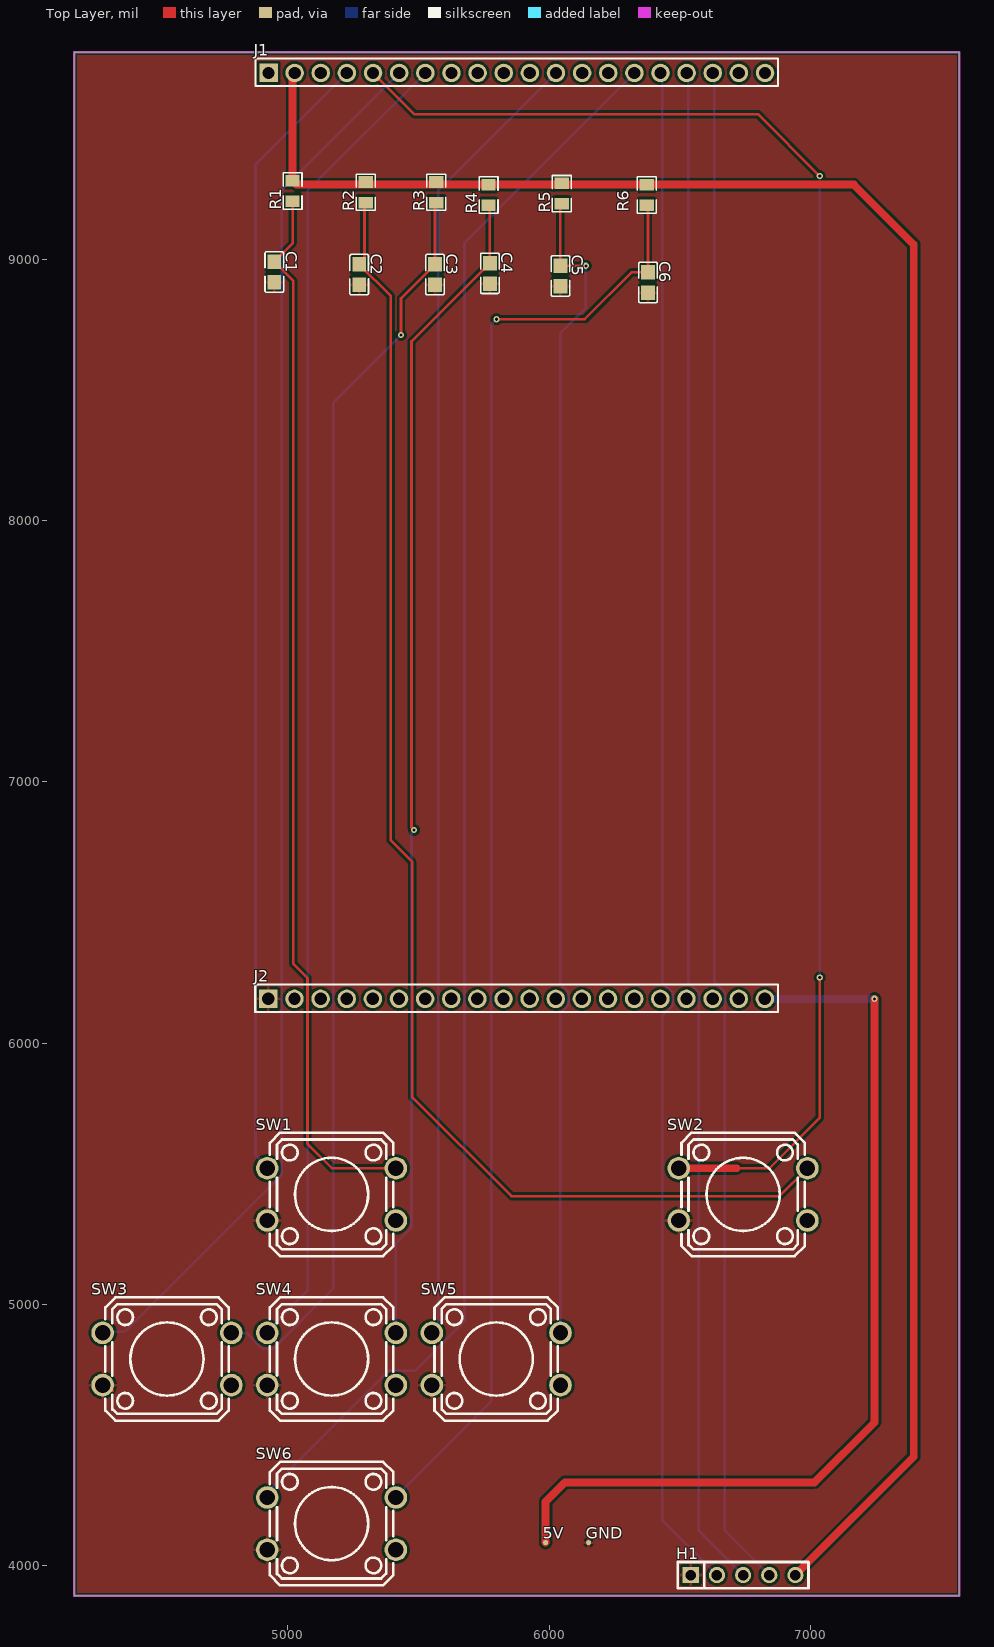
[diagram p0: Top Layer view]
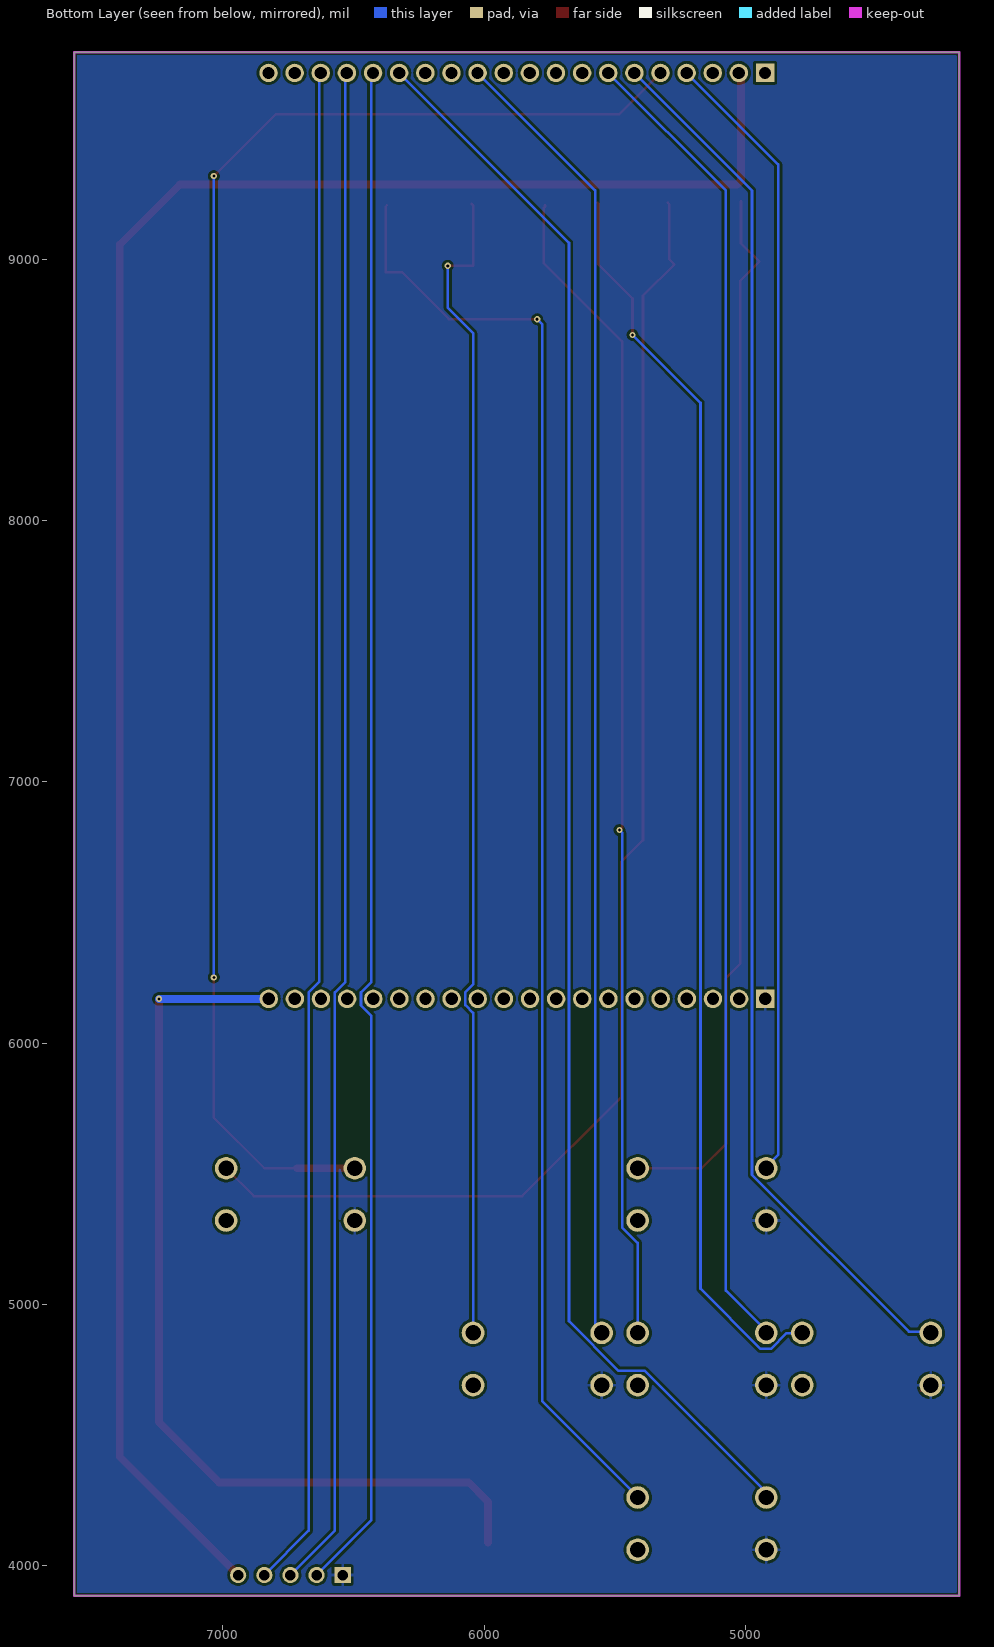
[diagram p1: Bottom Layer view, seen from below]
# Altium PCB MISC51976.pcbdoc
Units mil, origin at the board's own origin, x right, y up, seen from the top; angles counter-clockwise.
Board outline 3385.83 x 5905.51 mil, 2 copper layers (Top Layer, Bottom Layer), stack 62.206 mil thick; 23 components, 18 nets, 95 pads, 7 vias.

## Layer stack, top to bottom
Top Solder Mask Layer: solder mask 0.394, Dk 3.3
Top Layer: signal copper 1.379
Dielectric1: surface 59.449, FR4, Dk 4.5
Bottom Layer: signal copper 1.378
Bottom Solder Mask Layer: solder mask 0.394, Dk 3.3

## Board outline
4182.8,9791.97 4182.8,3886.46 7568.63,3886.46 7568.63,9791.97

## Design rules (kind name [scope] priority, off if disabled: settings)
BoardOutlineClearance copperThickness2oz_1 [All] p2 off: genericclearance=7.99 ignorepadtopadclearanceinfootprint=FALSE except(0: Arc-SplitContinuation Track-SplitContinuation SMDPad-SplitContinuation THPad-SplitContinuation Via-SplitContinuation Fill-SplitContinuation Region-SplitContinuation Poly-SplitContinuation Text-SplitContinuation Hole-SplitContinuation; 5.98: Arc-CutoutEdge SMDPad-CutoutEdge THPad-CutoutEdge Via-CutoutEdge Fill-CutoutEdge Region-CutoutEdge Text-CutoutEdge; 6.93: Hole-OutlineEdge Hole-CutoutEdge; 10: Poly-OutlineEdge Poly-CutoutEdge; 11.81: Arc-OutlineEdge Track-OutlineEdge SMDPad-OutlineEdge THPad-OutlineEdge Via-OutlineEdge Fill-OutlineEdge Region-OutlineEdge Text-OutlineEdge Track-CutoutEdge)
BoardOutlineClearance copperThickness1oz_1 [All] p4: genericclearance=4.02 ignorepadtopadclearanceinfootprint=FALSE except(0: Arc-SplitContinuation Track-SplitContinuation SMDPad-SplitContinuation THPad-SplitContinuation Via-SplitContinuation Fill-SplitContinuation Region-SplitContinuation Poly-SplitContinuation Text-SplitContinuation Hole-SplitContinuation; 6: SMDPad-CutoutEdge THPad-CutoutEdge Via-CutoutEdge Fill-CutoutEdge Region-CutoutEdge Text-CutoutEdge; 6.93: Hole-OutlineEdge Hole-CutoutEdge; 10: Poly-OutlineEdge Poly-CutoutEdge; 11.8: Arc-OutlineEdge Track-OutlineEdge SMDPad-OutlineEdge THPad-OutlineEdge Via-OutlineEdge Fill-OutlineEdge Region-OutlineEdge Text-OutlineEdge; 11.81: Arc-CutoutEdge Track-CutoutEdge)
Clearance copperThickness2oz [All] p1 off: gap=7.99 ignorepadtopadclearanceinfootprint=FALSE except(5.98: SMDPad-Track SMDPad-SMDPad THPad-Track SMDPad-THPad THPad-THPad Track-Via SMDPad-Via THPad-Via Via-Via Fill-Track Region-Track Fill-SMDPad Region-SMDPad Fill-THPad Region-THPad Fill-Via Region-Via Fill-Fill Fill-Region Region-Region Arc-Track Arc-SMDPad Arc-THPad Arc-Via Fill-Arc Region-Arc Arc-Arc Text-Track SMDPad-Text Text-THPad Text-Via Fill-Text Region-Text Arc-Text Text-Text; 6.93: Hole-Track Hole-SMDPad Hole-THPad Hole-Via Fill-Hole Region-Hole Hole-Arc Hole-Text; 10: Poly-Track Poly-SMDPad Poly-THPad Poly-Via Poly-Fill Poly-Region Poly-Poly Poly-Arc Poly-Text Poly-Hole)
Clearance copperThickness1oz [All] p3: gap=4.02 ignorepadtopadclearanceinfootprint=FALSE except(5.98: SMDPad-Track SMDPad-SMDPad THPad-Track SMDPad-THPad THPad-THPad Track-Via SMDPad-Via THPad-Via Via-Via Fill-Track Region-Track Fill-SMDPad Region-SMDPad Fill-THPad Region-THPad Fill-Via Region-Via Fill-Fill Fill-Region Region-Region; 6: Arc-Track Arc-SMDPad Arc-THPad Arc-Via Fill-Arc Region-Arc Arc-Arc Text-Track SMDPad-Text Text-THPad Text-Via Fill-Text Region-Text Arc-Text Text-Text; 6.93: Hole-Track Hole-SMDPad Hole-THPad Hole-Via Fill-Hole Region-Hole Hole-Arc Hole-Text; 10: Poly-Track Poly-SMDPad Poly-THPad Poly-Via Poly-Fill Poly-Region Poly-Poly Poly-Arc Poly-Text Poly-Hole)
DiffPairsRouting differentialPair [All] p1: maxlimit=6 minlimit=6 mostfreqgap=6 toplayer_minwidth=5 toplayer_prefwidth=10 toplayer_maxwidth=100 toplayer_mingap=6 toplayer_prefgap=6 toplayer_maxgap=6 bottomlayer_minwidth=5 bottomlayer_prefwidth=10 bottomlayer_maxwidth=100 bottomlayer_mingap=6 bottomlayer_prefgap=6 bottomlayer_maxgap=6 maxuncoupledlength=10
HoleToHoleClearance otherClearance [All] p1: gap=11.81 allowstackedmicrovias=TRUE
Length netLength [All] p1: minlimit=0 maxlimit=0
MatchedLengths netLengthTolerance [All] p1: tolerance=1000
PasteMaskExpansion pasteMaskExpansion [All] p1: expansion=0
PlaneConnect innerPlane [All] p1: planeconnectstyle=Relief reliefexpansion=20 reliefentries=4 reliefconductorwidth=10 reliefairgap=10
PolygonConnect copperRegion [(InNet('GND'))] p1: connectstyle=Relief reliefconductorwidth=10 reliefentries=4 polygonreliefangle="90 Angle" airgapwidth=10 via.connectstyle=Relief via.reliefconductorwidth=10 via.reliefentries=4 via.polygonreliefangle="90 Angle" via.airgapwidth=10
RoutingVias viaSize [All] p1: holewidth=12.01 width=24.02 viastyle="Through Hole" minholewidth=11.81 minwidth=19.68 maxholewidth=248.03 maxwidth=393.7
SolderMaskExpansion solderMaskExpansion [IsVia] p1: expansion=-1000 istentingtop=TRUE
SolderMaskExpansion solderMaskExpansion [All] p2: expansion=2 istentingtop=FALSE
Width copperThickness2oz_2 [All] p1 off: maxlimit=100 minlimit=8 preferedwidth=10
Width copperThickness1oz_2 [All] p2: maxlimit=100 minlimit=5 preferedwidth=10

## Components (designator, comment, footprint, x,y, rotation, side; value= is the part's Value field where it differs from the comment)
5V "" Test-Point-0.5mm 5985.89,4089.52 r0 top
C1 "100nF" C0805 4947.8,8951.46 r270 top
C2 "100nF" C0805 5272.8,8941.46 r270 top
C3 "100nF" C0805 5562.8,8941.46 r270 top
C4 "100nF" C0805 5772.8,8946.46 r270 top
C5 "100nF" C0805 6042.8,8936.46 r270 top
C6 "100nF" C0805 6377.8,8911.46 r270 top
GND "" Test-Point-0.5mm 6150.26,4089.52 r0 top
H1 "2.54-1*5P母" HDR-TH_5P-P2.54-V-F 6741.85,3965.19 r0 top
J1 "2.54-1*20P直针" HDR-TH_20P-P2.54-V-M-1 5875.73,9713.23 r0 top
J2 "2.54-1*20P直针" HDR-TH_20P-P2.54-V-M-1 5875,6170 r0 top
R1 "10kΩ" R0805 5017.8,9261.46 r90 top
R2 "10kΩ" R0805 5297.8,9256.46 r90 top
R3 "10kΩ" R0805 5567.8,9256.46 r90 top
R4 "10kΩ" R0805 5767.8,9246.46 r90 top
R5 "10kΩ" R0805 6047.8,9251.46 r90 top
R6 "10kΩ" R0805 6372.8,9246.46 r90 top
SW1 "TC-1103-C-K" KEY-TH_4P-L12.0-W12.0-P5.00-LS12.5 5167.05,5421.89 r0 top
SW2 "TC-1103-C-K" KEY-TH_4P-L12.0-W12.0-P5.00-LS12.5 6741.86,5421.88 r0 top
SW3 "TC-1103-C-K" KEY-TH_4P-L12.0-W12.0-P5.00-LS12.5 4537.13,4791.97 r0 top
SW4 "TC-1103-C-K" KEY-TH_4P-L12.0-W12.0-P5.00-LS12.5 5167.07,4791.96 r0 top
SW5 "TC-1103-C-K" KEY-TH_4P-L12.0-W12.0-P5.00-LS12.5 5796.97,4791.97 r0 top
SW6 "TC-1103-C-K" KEY-TH_4P-L12.0-W12.0-P5.00-LS12.5 5167.07,4162.04 r0 top

## Footprints (in the part's own frame and the unit in brackets; to place one, negate y for a bottom-side part, rotate by r counter-clockwise, add the part's x,y. Pads: shape width x height; smd on the part's side, far side on the other; paste and mask are expansions set on the pad)
C0805 [mm]
  rect 1.41x1.35 smd paste-100 mask+0.051: 1(-1,0) 2(1,0)
  silkscreen extent -1.96,-0.9 1.96,0.9
HDR-TH_5P-P2.54-V-F [mil]
  rect 62x62 hole 40.16: 1(-200,0)
  round 62 hole 40.16: 2(-100,0) 3(0,0) 4(100,0) 5(200,0)
  silkscreen extent -250,-50 250,50
HDR-TH_20P-P2.54-V-M-1 [mm]
  rect 1.8x1.8 hole 1.2: 1(-24.13,0)
  round 1.8 hole 1.2: 2(-21.59,0) 3(-19.05,0) 4(-16.51,0) 5(-13.97,0) 6(-11.43,0) 7(-8.89,0) 8(-6.35,0) 9(-3.81,0) 10(-1.27,0) 11(1.27,0) 12(3.81,0) 13(6.35,0) 14(8.89,0) 15(11.43,0) 16(13.97,0) 17(16.51,0) 18(19.05,0) 19(21.59,0) 20(24.13,0)
  silkscreen extent -25.4,-1.27 25.4,1.4
KEY-TH_4P-L12.0-W12.0-P5.00-LS12.5 [mil]
  round 86.6 hole 59.1 paste+0 mask+2: 1(-246.1,100) 2(246.1,100) 3(-246.1,-100) 4(246.1,-100)
  silkscreen extent -236,-236 236,236
R0805 [mm]
  rect 1.133x1.377 smd paste-100 mask+0.051: 1(-1,0) 2(1,0)
  silkscreen extent -1.76,-0.92 1.76,0.92
Test-Point-0.5mm [mm]
  round 0.5 smd: 1(0,0)

## Via types
v1: diameter 24.02, hole 12, Top Layer to Bottom Layer, 7 vias

## Nets (pads, with @x,y where several pads share a name; then routed paths per layer and width w, separated by ;. In a path a pad name is that pad's centre, name@x,y a point inside that pad or via, vN(x,y) a via of type N, cw(c..) or ccw(c..) an arc to the next point about the centre after c; other vN are vias at no path point)
$1N52: C3.1 R3.1 SW3.2 | length 4829.3
  Top Layer w10: v1(5432.8,8710.83) 5432.8,8850.83 C3.1 5562.8,9210.83 R3.1
  Bottom Layer w10: SW3.2 4792.8,4890.84 4842.8,4890.84 4902.8,4830.84 4942.8,4830.84 5172.8,5060.84 5172.8,8450.83 v1(5432.8,8710.83)
$1N57: C4.1 R4.1 SW4.2 | length 4474.6
  Top Layer w10: v1(5482.8,6815.84) 5472.8,6825.84 5472.8,8685.83 C4.1 5772.8,9195.83 5767.8,9200.83 R4.1
  Bottom Layer w10: SW4.2 5412.8,4895.84 5412.8,5235.84 5472.8,5295.84 5472.8,6805.84 v1(5482.8,6815.84)
$1N101: C1.1 R1.1 SW1.2 | length 4065.5
  Top Layer w10: R1.1 5017.8,9060.83 C1.1 5020,8918.63 5020,6305 5075,6250 5075,5615 5168.11,5521.89 SW1.2
$1N104: C6.1 R6.1 SW6.2 | length 5580.7
  Top Layer w10: v1(5797.8,8770.84) 6135.84,8770.84 6315.83,8950.83 C6.1 6377.8,9200.83 R6.1
  Bottom Layer w10: SW6.2 5413.17,4266.21 5778.58,4631.62 5778.58,8751.62 v1(5797.8,8770.84)
$1N106: C5.1 R5.1 SW5.2 | length 4484.9
  Top Layer w10: R5.1 6042.8,9205.83 C5.1 ; v1(6140,8975) C5.1@6043.63,8975 ; C5.1 C5.1@6043.63,8975 ; C5.1 C5.1@6043.63,8975
  Bottom Layer w10: SW5.2 6042.8,4895.84 6042.8,6115.84 6072.8,6145.84 6072.8,6195.84 6042.8,6225.84 6042.8,8717.8 6140,8815 v1(6140,8975)
$1N108: C2.1 R2.1 SW2.2 | length 5230.5
  Top Layer w10: R2.1 5292.8,9210.83 5292.8,9000.83 C2.1 5392.8,8860.83 5392.8,6920.27 5392.8,6777.2 5475,6695 5475,5795 5855,5415 6881.08,5415 SW2.2
+3.3V: H1.5 J1.2 R1.2 R2.2 R3.2 R4.2 R5.2 R6.2 | length 8173
  Top Layer w30: J1.2 5017.8,9705.3 R1.2 5032.8,9285.83 R4.2 R6.2 7165.54,9285.83 7395,9056.37 7395,4418.34 H1.5
+5V: 5V.1 J2.20 | length 3581.4
  Top Layer w30: 5V.1 5985.89,4245.89 6060,4320 7015,4320 7245,4550 v1(7245,6170)
  Bottom Layer w30: J2.20 v1(7245,6170)
GND: C1.2 C2.2 C3.2 C4.2 C5.2 C6.2 GND.1 H1.1 J2.1 SW1.3 SW2.3 SW3.3 SW4.3 SW5.3 SW6.3 | length 73.3
  Top Layer w10: SW3.3@4272.8,4711.46 4314,4670.26 4329,4670.26
IO4: J1.4 SW1.1 | length 4355
  Bottom Layer w10: SW1.1 4920.95,5528.02 4875.73,5573.24 4875.73,9363.23 J1.4
IO5: J1.5 SW2.1 | length 6095.7
  Top Layer w10: J1.5 5483.1,9555.86 6797.96,9555.86 v1(7035,9318.82) ; 6716.88,5521.88 6841.88,5521.88 7035,5715 v1(7035,6252.09)
  Top Layer w30: SW2.1 6716.88,5521.88
  Bottom Layer w10: v1(7035,6252.09) v1(7035,9318.82)
IO6: J1.6 SW3.1 | length 5338.1
  Bottom Layer w10: SW3.1 4295.73,4896.67 4375.73,4896.67 4975.73,5496.67 4975.73,9263.23 J1.6
IO7: J1.7 SW4.1 | length 5071.8
  Bottom Layer w10: SW4.1 4920.97,4898.48 5075.73,5053.24 5075.73,9263.23 J1.7
IO8: J1.12 SW5.1 | length 5018
  Bottom Layer w10: SW5.1 5550.87,4898.38 5575.73,4923.24 5575.73,9263.23 J1.12
IO9: J1.15 SW6.1 | length 6091.6
  Bottom Layer w10: SW6.1 4925.73,4266.81 4925.73,4286.81 5385.73,4746.8 5485.73,4746.8 5675.73,4936.8 5675.73,9063.23 J1.15
IO10: H1.2 J1.16 | length 5870.2
  Bottom Layer w10: J1.16 6431.85,9705.18 6431.85,6235.19 6471.85,6195.19 6471.85,6145.19 6431.85,6105.19 6431.85,4175.19 H1.2@6641.85,3965.19
IO11: H1.3 J1.17 | length 5837.1
  Bottom Layer w10: J1.17 6531.85,9705.18 6531.85,6235.19 6571.85,6195.19 6571.85,4135.19 H1.3@6741.85,3965.19
IO12: H1.4 J1.18 | length 5837.1
  Bottom Layer w10: J1.18 6631.85,9705.18 6631.85,6235.19 6671.85,6195.19 6671.85,4135.19 H1.4@6841.85,3965.19
pads on no net: J1.1 J1.3 J1.8 J1.9 J1.10 J1.11 J1.13 J1.14 J1.19 J1.20 J2.2 J2.3 J2.4 J2.5 J2.6 J2.7 J2.8 J2.9 J2.10 J2.11 J2.12 J2.13 J2.14 J2.15 J2.16 J2.17 J2.18 J2.19 SW1.4 SW2.4 SW3.4 SW4.4 SW5.4 SW6.4

## Polygon pours and split planes (outlines as drawn)
GND on Top Layer (solid, remove dead copper, pour order 0): 3000,10425 3000,3000 8200,3000 8200,10425
GND on Bottom Layer (solid, remove dead copper, pour order 2): 3905,9995 3905,3085 8300,3085 8300,9995

## Keep-outs
Board Outline Layer:
  the board outline again, w10